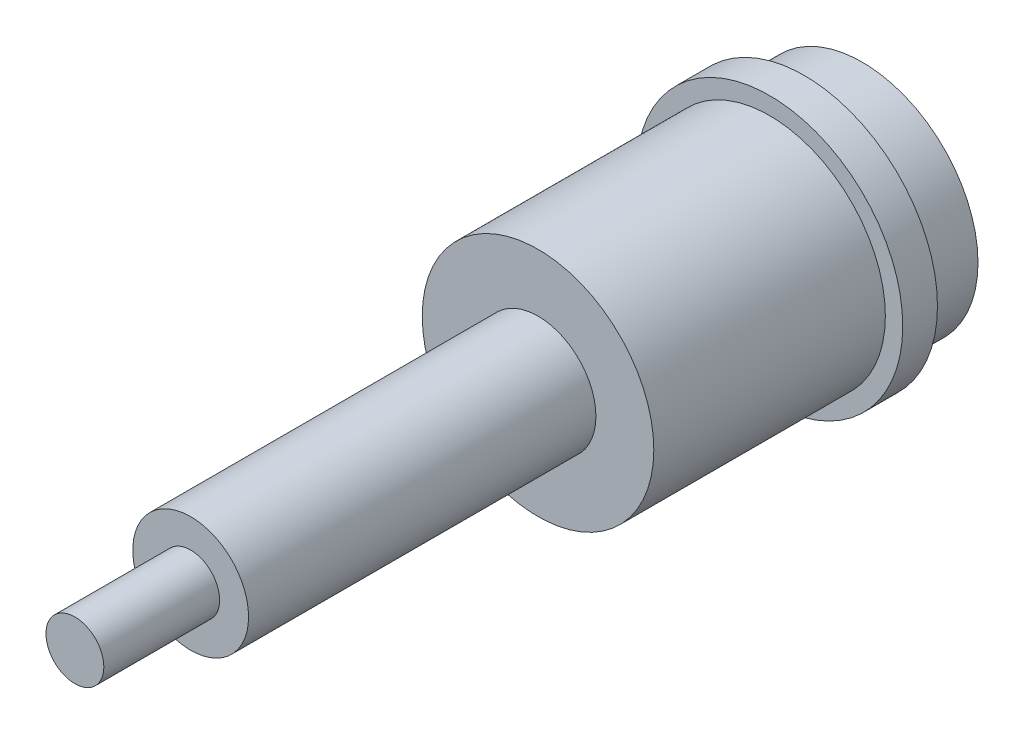
SolidWorks part; units mm, degrees
ref_plane "Front Plane" through (0, 0, 0) normal (0, 0, 1) x (1, 0, 0)
ref_plane "Top Plane" through (0, 0, 0) normal (0, 1, 0) x (1, 0, 0)
ref_plane "Right Plane" through (0, 0, 0) normal (1, 0, 0) x (0, 0, -1)
other "Configuration Table"
sketch "Sketch1" plane through (0, 0, 0) normal (0, 0, 1) x (1, 0, 0)
  circle A0 centre (0, 0) radius 10
  dimension "D1" = 20
extrude "Boss-Extrude1" add sketch "Sketch1" along normal blind 5
sketch "Sketch2" plane through (0, 0, 5) normal (0, 0, 1) x (1, 0, 0)
  circle A0 centre (0, 0) radius 11.5
  dimension "D1" = 23
extrude "Boss-Extrude2" add sketch "Sketch2" along normal blind 3
sketch "Sketch3" plane through (0, 0, 8) normal (0, 0, 1) x (1, 0, 0)
  circle A0 centre (0, 0) radius 10
  dimension "D1" = 20
extrude "Boss-Extrude3" add sketch "Sketch3" along normal blind 20
sketch "Sketch4" plane through (0, 0, 28) normal (0, 0, 1) x (1, 0, 0)
  circle A0 centre (0, 0) radius 5
  dimension "15" = 10
extrude "Boss-Extrude4" add sketch "Sketch4" along normal blind 30
sketch "Sketch5" plane through (0, 0, 58) normal (0, 0, 1) x (1, 0, 0)
  circle A0 centre (0, 0) radius 2.5
  dimension "D1" = 5
extrude "Boss-Extrude5" add sketch "Sketch5" along normal blind 10
cosmetic thread "Cosmetic Thread1" parameters "D1"=5, "D2"=4.134
